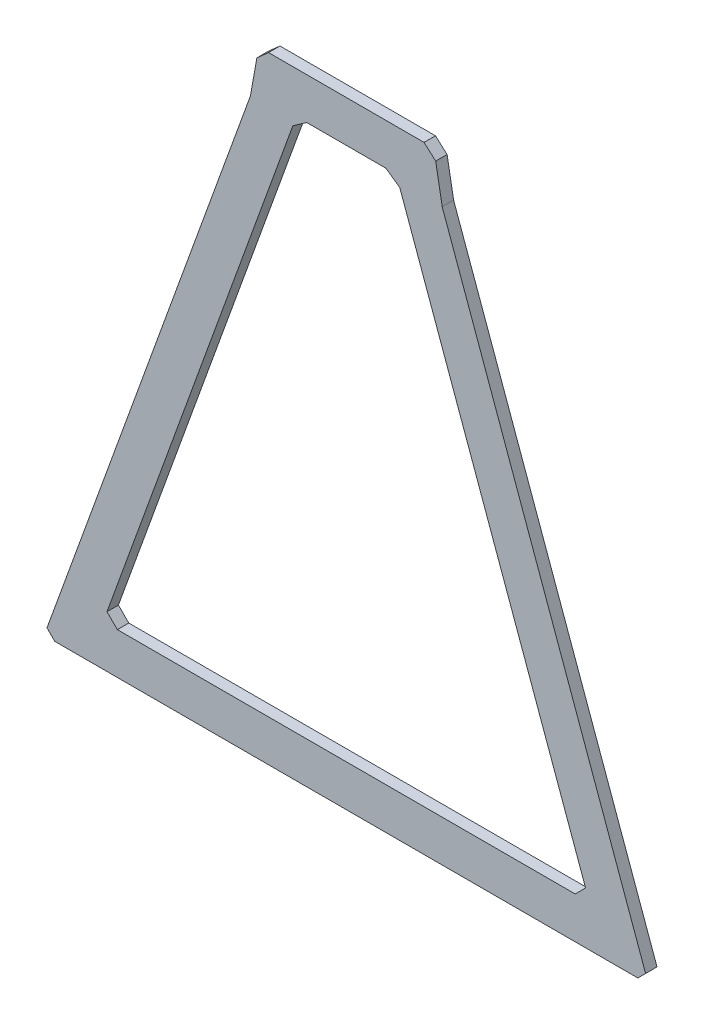
SolidWorks part; units mm, degrees
material "普通碳钢"
ref_plane "Front Plane" through (0, 0, 0) normal (0, 0, 1) x (1, 0, 0)
ref_plane "Top Plane" through (0, 0, 0) normal (0, 1, 0) x (1, 0, 0)
ref_plane "Right Plane" through (0, 0, 0) normal (1, 0, 0) x (0, 0, -1)
sketch "Sketch1" plane through (0, 0, 0) normal (0, 0, 1) x (1, 0, 0)
  line L0 (0, 0) -> (0, 843.7522) construction
  line L1 (0, 0) -> (357.1875, 0)
  line L2 (366.7125, 9.525) -> (117.475, 698.5)
  line L3 (117.475, 698.5) -> (109.5375, 742.95)
  line L4 (95.25, 755.65) -> (0, 755.65)
  line L5 (357.1875, 0) -> (366.7125, 9.525)
  line L6 (95.25, 755.65) -> (109.5375, 742.95)
  line L7 (-280.4652, 50.8) -> (280.4652, 50.8)
  line L8 (-65.4763, 692.9074) -> (-48.4561, 704.85)
  line L9 (293.1652, 63.5) -> (65.4763, 692.9074)
  line L10 (297.7594, 50.8) -> (68.2288, 685.2988) construction
  line L11 (64.7375, 704.85) -> (64.7375, 704.85)
  line L12 (48.4561, 704.85) -> (-48.4561, 704.85)
  line L13 (68.2288, 685.2988) -> (64.7375, 704.85) construction
  line L14 (64.7375, 704.85) -> (0, 704.85) construction
  line L15 (65.4763, 692.9074) -> (48.4561, 704.85)
  line L16 (0, 50.8) -> (297.7594, 50.8) construction
  line L17 (280.4652, 50.8) -> (293.1652, 63.5)
  line L18 (297.7594, 50.8) -> (297.7594, 50.8) construction
  line L19 (-293.1652, 63.5) -> (-65.4763, 692.9074)
  line L20 (-280.4652, 50.8) -> (-293.1652, 63.5)
  line L21 (0, 0) -> (-357.1875, 0)
  line L22 (-357.1875, 0) -> (-366.7125, 9.525)
  line L23 (-366.7125, 9.525) -> (-117.475, 698.5)
  line L24 (-117.475, 698.5) -> (-109.5375, 742.95)
  line L25 (-95.25, 755.65) -> (-109.5375, 742.95)
  line L26 (-95.25, 755.65) -> (0, 755.65)
  point P16 (61.1561, 704.85)
  dimension "D1" = 9.525
  dimension "D2" = 714.375
  dimension "D3" = 733.425
  dimension "D4" = 742.95
  dimension "D5" = 698.5
  dimension "D6" = 190.5
  dimension "D7" = 219.075
  dimension "D8" = 234.95
  dimension "D9" = 755.65
  dimension "D10" = 50.8
  dimension "D11" = 12.7
  dimension "D12" = 135
extrude "Boss-Extrude1" add sketch "Sketch1" along normal blind 14 contours L26 L25 L24 L23 L22 L21 L1 L5 L2 L3 L6 L4 L7 L20 L19 L8 L12 L15 L9 L17
